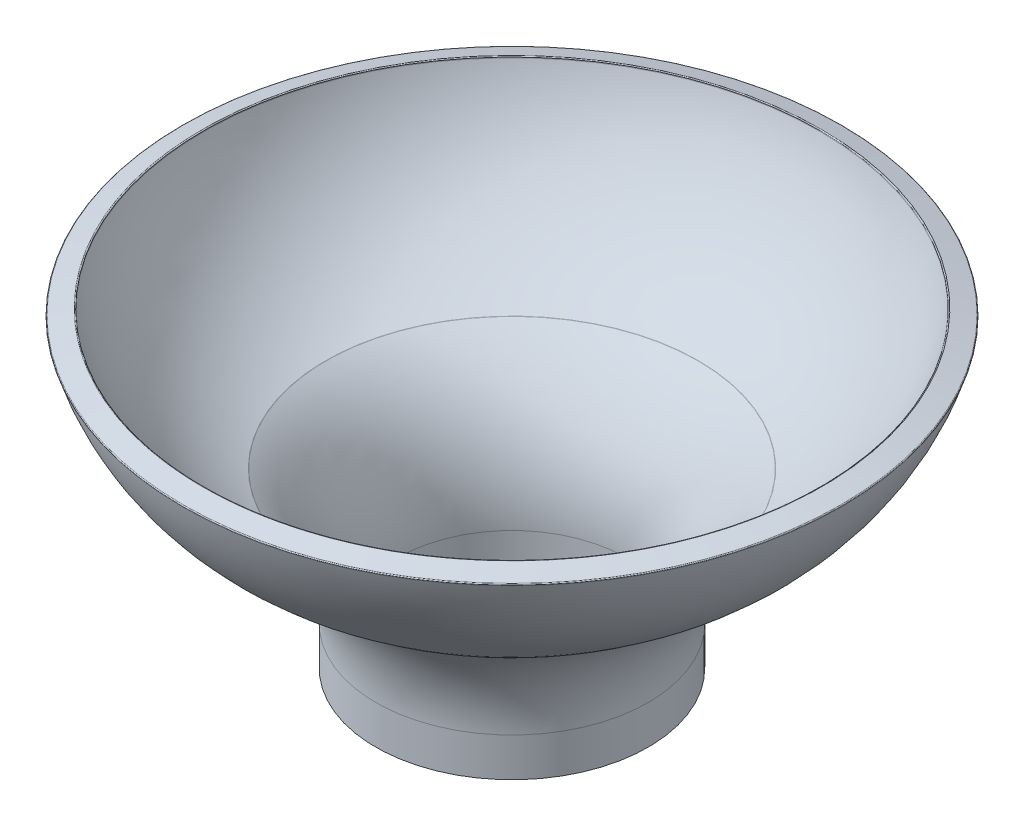
from build123d import *


with BuildPart() as part:
    # Sketch1 → Revolution1 (revolve)
    with BuildSketch(Plane.XY, mode=Mode.PRIVATE) as revolution1_sk:
        with BuildLine():
            Line((31.832021846, -49.650440399), (31.832021846, -37.325883541))
            ThreePointArc((31.832021846, -37.325883541), (25.751638451, -13.050886085), (8.946333163, 5.491721011))
            ThreePointArc((8.946333163, 5.491721011), (8.909163165, 5.51428476), (8.870173321, 5.533533751))
            ThreePointArc((8.870173321, 5.533533751), (-15.299365519, 23.173876843), (-29.894384958, 49.29539517))
            Line((-29.894384958, 49.29539517), (-29.952363221, 49.486793945))
            ThreePointArc((-29.952363221, 49.486793945), (-30.097956714, 49.664342007), (-30.326452298, 49.686937298))
            Line((-30.326452298, 49.686937298), (-36.451598229, 47.831516233))
            ThreePointArc((-36.451598229, 47.831516233), (-36.62914629, 47.685922739), (-36.651741582, 47.457427155))
            Line((-36.651741582, 47.457427155), (-36.593763319, 47.266028379))
            ThreePointArc((-36.593763319, 47.266028379), (-20.737303749, 18.756830634), (5.500318761, -0.628442931))
            ThreePointArc((5.500318761, -0.628442931), (19.703559865, -16.586929303), (24.832021846, -37.325883541))
            Line((24.832021846, -37.325883541), (24.832021846, -49.650440399))
            Line((24.832021846, -49.650440399), (31.832021846, -49.650440399))
        make_face()
    revolve(revolution1_sk.sketch.rotate(Axis((68.222021846, -49.650440399, 0), (0, 1, 0)), 270), axis=Axis((68.222021846, -49.650440399, 0), (0, 1, 0)))


solid = part.part
